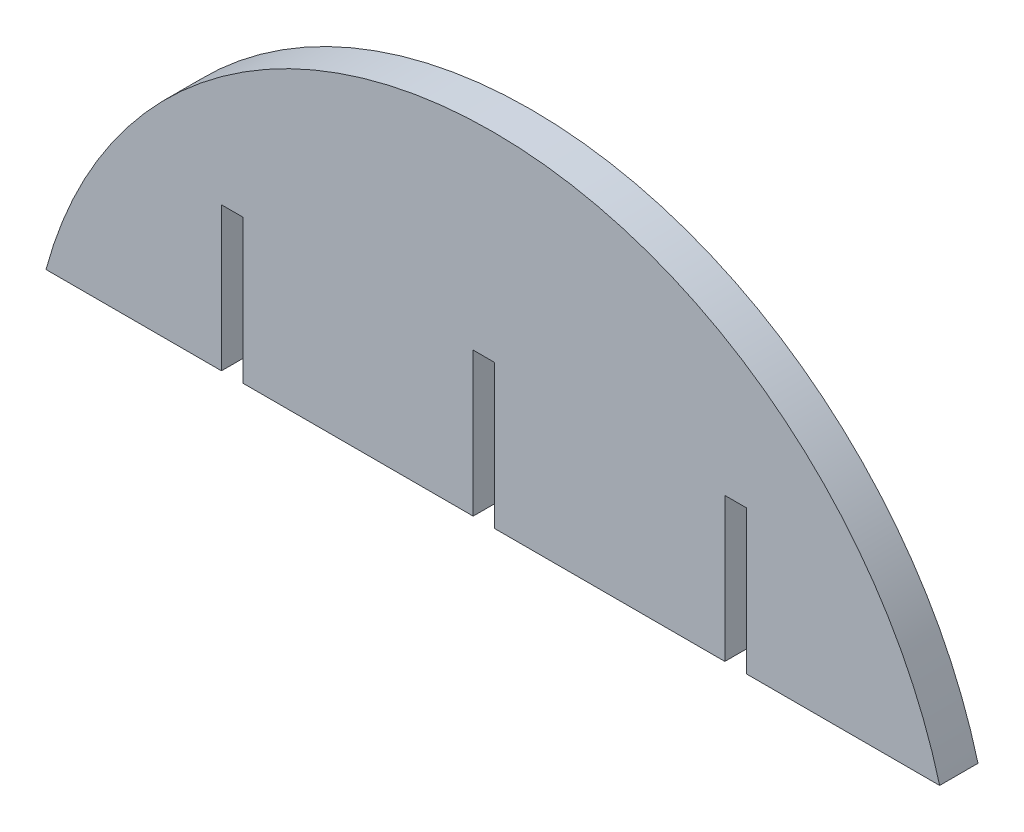
from build123d import *

# Parameters (mm, degrees)
BOSS_EXTRUDE1_DEPTH = 8
CUT_EXTRUDE1_DEPTH  = 10
SKETCH3_W           = 4.5
SKETCH3_H           = 30
CUT_EXTRUDE2_DEPTH  = 10


with BuildPart() as part:
    # Sketch1 → Boss-Extrude1 (new body)
    with BuildSketch(Plane.XY):
        with BuildLine():
            Line((-94.65, 0), (98.35, 0))
            ThreePointArc((98.35, 0), (1.85, 96.5), (-94.65, 0))
        make_face()
    extrude(amount=BOSS_EXTRUDE1_DEPTH)

    # Sketch2 → Cut-Extrude1 (cut)
    with BuildSketch(Plane.XY.offset(8)):
        Polygon((-94.65, 0), (-94.65, 25), (109.452328138, 25), (98.649241205, -24.174377991), align=None)
    extrude(amount=-CUT_EXTRUDE1_DEPTH, mode=Mode.SUBTRACT)

    # Sketch3 → Cut-Extrude2 (cut)
    with BuildSketch(Plane(origin=(0, 0, 0), x_dir=(-1, 0, 0), z_dir=(0, 0, -1))):
        with Locations((0, 40)):
            Rectangle(SKETCH3_W, SKETCH3_H)
        with Locations((52.5, 40)):
            Rectangle(SKETCH3_W, SKETCH3_H)
        with Locations((-52.5, 40)):
            Rectangle(SKETCH3_W, SKETCH3_H)
    extrude(amount=-CUT_EXTRUDE2_DEPTH, mode=Mode.SUBTRACT)


solid = part.part
